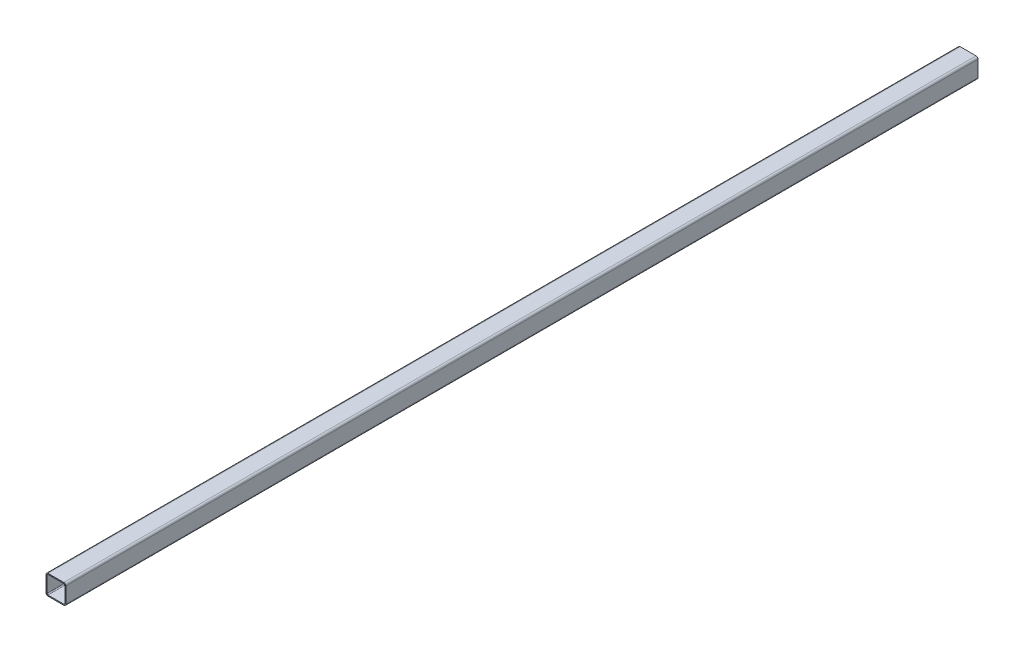
from build123d import *

# Parameters (mm, degrees)
BOSS_EXTRUDE1_DEPTH = 4600


with BuildPart() as part:
    # Sketch1 → Boss-Extrude1 (new body)
    with BuildSketch(Plane.XY):
        with BuildLine():
            Line((10, 0), (90, 0))
            ThreePointArc((90, 0), (97.071067812, 2.928932188), (100, 10))
            Line((100, 10), (100, 90))
            ThreePointArc((100, 90), (97.071067812, 97.071067812), (90, 100))
            Line((90, 100), (10, 100))
            ThreePointArc((10, 100), (2.928932188, 97.071067812), (0, 90))
            Line((0, 90), (0, 10))
            ThreePointArc((0, 10), (2.928932188, 2.928932188), (10, 0))
        make_face()
        with BuildLine():
            Line((10, 95), (90, 95))
            ThreePointArc((90, 95), (93.535533906, 93.535533906), (95, 90))
            Line((95, 90), (95, 10))
            ThreePointArc((95, 10), (93.535533906, 6.464466094), (90, 5))
            Line((90, 5), (10, 5))
            ThreePointArc((10, 5), (6.464466094, 6.464466094), (5, 10))
            Line((5, 10), (5, 90))
            ThreePointArc((5, 90), (6.464466094, 93.535533906), (10, 95))
        make_face(mode=Mode.SUBTRACT)
    extrude(amount=BOSS_EXTRUDE1_DEPTH)


solid = part.part
